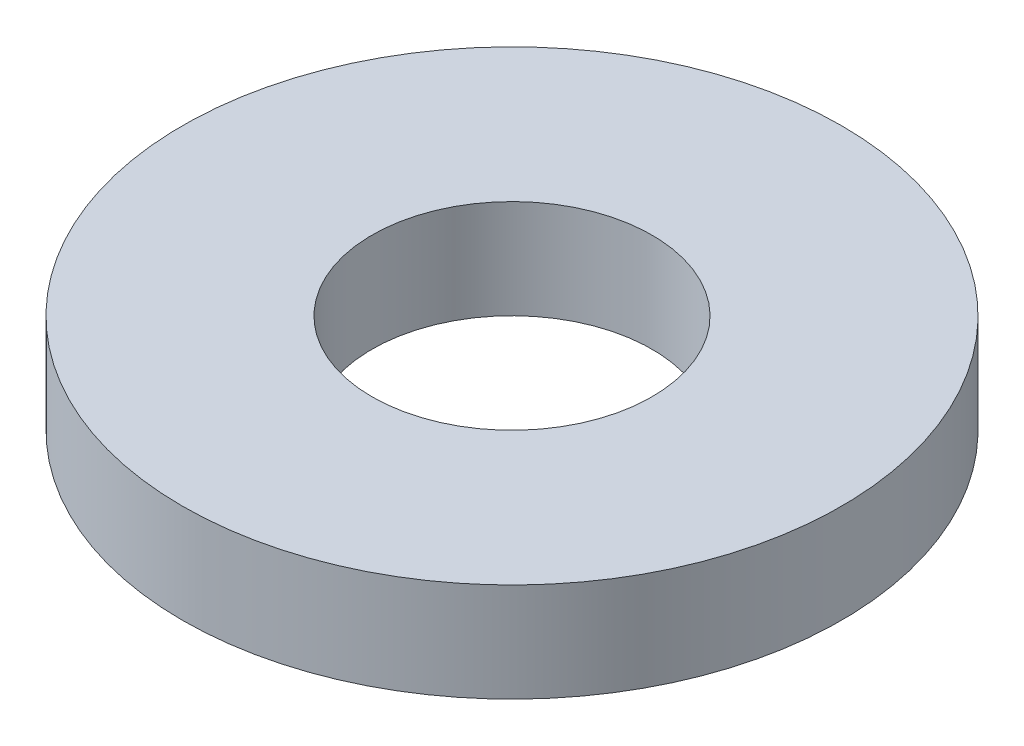
SolidWorks part; units mm, degrees
ref_plane "Front Plane" through (0, 0, 0) normal (0, 0, 1) x (1, 0, 0)
ref_plane "Top Plane" through (0, 0, 0) normal (0, 1, 0) x (1, 0, 0)
ref_plane "Right Plane" through (0, 0, 0) normal (1, 0, 0) x (0, 0, -1)
sketch "Sketch1" plane through (0, 0, 0) normal (0, 1, 0) x (1, 0, 0)
  circle A0 centre (0, 0) radius 4.25
  circle A1 centre (0, 0) radius 10
  dimension "D1" = 8.5
  dimension "D2" = 20
extrude "Boss-Extrude1" add sketch "Sketch1" along normal blind 3
